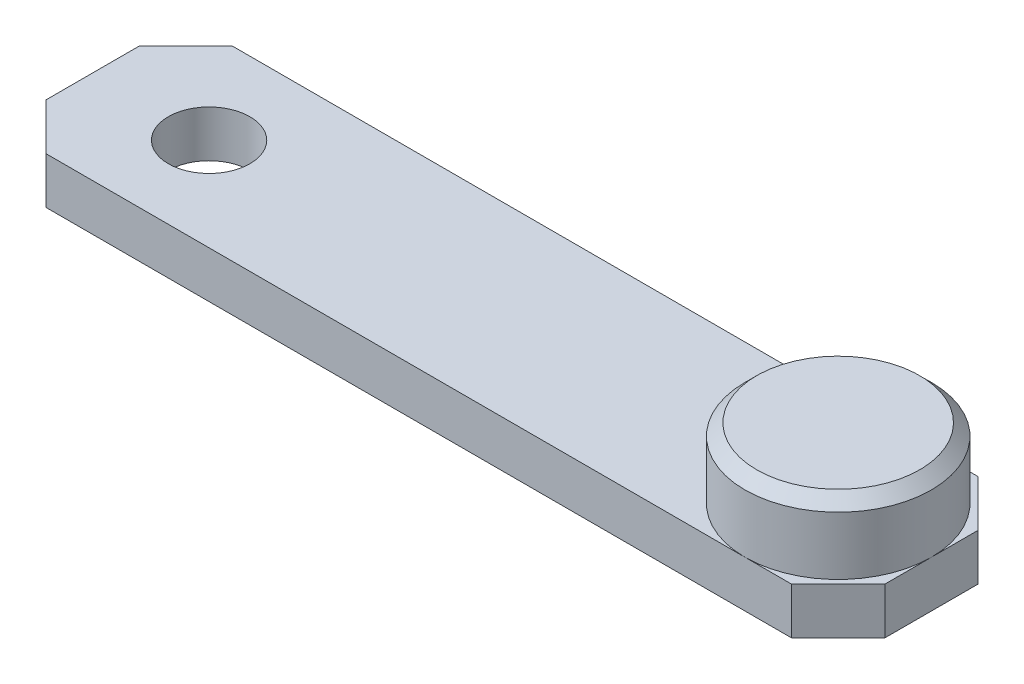
from build123d import *

# Parameters (mm, degrees)
SKETCH1_W           = 36
SKETCH1_H           = 8
BOSS_EXTRUDE1_DEPTH = 2
SKETCH2_R           = 1.75
CUT_EXTRUDE1_DEPTH  = 37.932370625
SKETCH3_R           = 4
BOSS_EXTRUDE2_DEPTH = 3
CHAMFER1_SIZE       = 0.5
CHAMFER2_SIZE       = 2


with BuildPart() as part:
    # Sketch1 → Boss-Extrude1 (new body)
    with BuildSketch(Plane(origin=(0, 0, 0), x_dir=(1, 0, 0), z_dir=(0, 1, 0))):
        with Locations((18, 4)):
            Rectangle(SKETCH1_W, SKETCH1_H)
    extrude(amount=BOSS_EXTRUDE1_DEPTH)

    # Sketch2 → Cut-Extrude1 (cut, through all)
    with BuildSketch(Plane(origin=(0, 2, 0), x_dir=(1, 0, 0), z_dir=(0, 1, 0))):
        with Locations(Location((5, 4, 0), (0, 0, 270))):
            Circle(SKETCH2_R)
    extrude(amount=-CUT_EXTRUDE1_DEPTH, mode=Mode.SUBTRACT)

    # Sketch3 → Boss-Extrude2 (add)
    with BuildSketch(Plane(origin=(0, 2, 0), x_dir=(1, 0, 0), z_dir=(0, 1, 0))):
        with Locations(Location((32, 4, 0), (0, 0, 270))):
            Circle(SKETCH3_R)
    extrude(amount=BOSS_EXTRUDE2_DEPTH)

    # Chamfer1
    chamfer1_edges = [part.edges().sort_by_distance(p)[0] for p in [
        (32, 5, -8),
    ]]
    chamfer(chamfer1_edges, length=CHAMFER1_SIZE)

    # Chamfer2
    chamfer2_edges = [part.edges().sort_by_distance(p)[0] for p in [
        (0, 1, -8),
        (36, 1, -8),
        (36, 1, 0),
        (0, 1, 0),
    ]]
    chamfer(chamfer2_edges, length=CHAMFER2_SIZE)


solid = part.part
